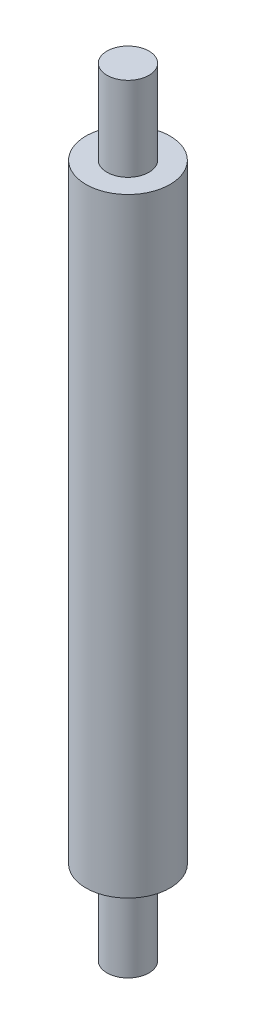
from build123d import *

# Parameters (mm, degrees)
CUT_EXTRUDE1_DEPTH = 2.5


with BuildPart() as part:
    # Sketch1 → Revolve1 (revolve)
    with BuildSketch(Plane(origin=(0, 0, 0), x_dir=(0, 0, -1), z_dir=(1, 0, 0))):
        Polygon((0, 185), (-10, 185), (-10, 145), (-20, 145), (-20, -145), (-10, -145), (-10, -185), (0, -185), align=None)
    revolve(axis=Axis((0, 189.929754582, 0), (0, -1, 0)))

    # Sketch2 → Cut-Extrude1 (cut)
    with BuildSketch(Plane(origin=(0, 0, -10), x_dir=(-1, 0, 0), z_dir=(0, 0, -1))):
        with BuildLine():
            Line((2.5, 175), (2.5, 155))
            ThreePointArc((2.5, 155), (0, 152.5), (-2.5, 155))
            Line((-2.5, 155), (-2.5, 175))
            ThreePointArc((-2.5, 175), (0, 177.5), (2.5, 175))
        make_face()
    cut_extrude1 = extrude(amount=-CUT_EXTRUDE1_DEPTH, mode=Mode.SUBTRACT)

    # Mirror1: Cut-Extrude1 across plane
    add(cut_extrude1.mirror(Plane.ZX), mode=Mode.SUBTRACT)


solid = part.part
